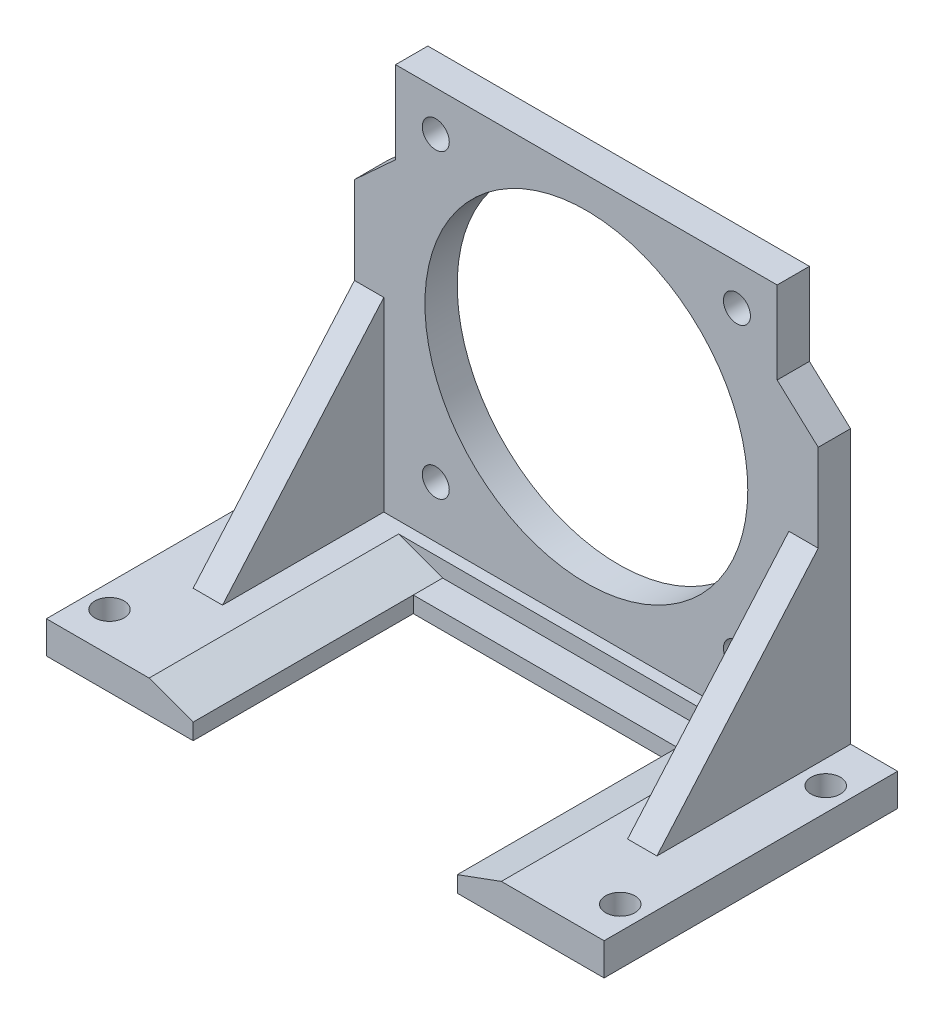
SolidWorks part; units mm, degrees
ref_plane "前视基准面" through (0, 0, 0) normal (0, 0, 1) x (1, 0, 0)
ref_plane "上视基准面" through (0, 0, 0) normal (0, 1, 0) x (1, 0, 0)
ref_plane "右视基准面" through (0, 0, 0) normal (1, 0, 0) x (0, 0, -1)
sketch "草图1" plane through (0, 0, 0) normal (0, 0, 1) x (1, 0, 0)
  line L0 (79, 24.1009) -> (79, 0)
  line L1 (65, -65) -> (-65, -65)
  line L2 (65, -65) -> (65, 65)
  line L3 (65, 65) -> (-65, 65)
  line L4 (-65, -65) -> (-65, 65)
  line L5 (65, -65) -> (-65, 65) construction
  line L6 (65, 65) -> (-65, -65) construction
  line L7 (-65, -65) -> (65, -65)
  line L8 (-65, -65) -> (-65, -69)
  line L9 (-65, -69) -> (65, -69)
  line L10 (65, -65) -> (65, -69)
  line L11 (-79, 0) -> (-79, -69)
  line L12 (-79, -69) -> (-65, -69)
  line L13 (0, 65) -> (0, -65) construction
  line L14 (79, -69) -> (65, -69)
  line L15 (65, 36.9502) -> (79, 24.1009)
  line L16 (79, 0) -> (79, -69)
  line L17 (-65, 36.9502) -> (-79, 24.1009)
  line L18 (-79, 24.1009) -> (-79, 0)
  circle A0 centre (0, -0.5) radius 55
  circle A1 centre (-51.3, 51.3) radius 4.6
  circle A2 centre (51.3, 51.3) radius 4.6
  circle A3 centre (51.3, -51.3) radius 4.6
  circle A4 centre (-51.3, -51.3) radius 4.6
  point P0 (0, 0)
  dimension "D3" = 68.5
  dimension "D4" = 9.2
  dimension "D5" = 102.6
  dimension "D6" = 4
  dimension "D8" = 110
  dimension "D1" = 130
  dimension "D2" = 130
  dimension "D7" = 158
extrude "凸台-拉伸1" add sketch "草图1" along normal mid plane 11
sketch "草图2" plane through (0, -69, 0) normal (0, -1, 0) x (1, 0, 0)
  line L0 (0, 31.1448) -> (0, -33.7851) construction
  line L1 (-95, -5.5432) -> (95, -5.5432)
  line L2 (-95, -5.5432) -> (-95, 94.4568)
  line L3 (-95, 94.4568) -> (-45, 94.4568)
  line L4 (95, -5.5432) -> (95, 94.4568)
  line L6 (-45, 94.4568) -> (-45, 19.4568)
  line L7 (-45, 19.4568) -> (45, 19.4568)
  line L8 (45, 94.4568) -> (45, 19.4568)
  line L9 (45, 94.4568) -> (95, 94.4568)
  circle A0 centre (-87, 80.9568) radius 5
  circle A1 centre (-87, 10.9568) radius 5
  circle A2 centre (87, 10.9568) radius 5
  circle A3 centre (87, 80.9568) radius 5
  dimension "D5" = 70
  dimension "D6" = 16.5
  dimension "D7" = 10
  dimension "D8" = 174
  dimension "D1" = 190
  dimension "D2" = 100
  dimension "D3" = 90
  dimension "D4" = 25
extrude "凸台-拉伸2" add sketch "草图2" along normal blind 11
ref_plane "基准面1" through (74, 0, 0) normal (1, 0, 0) x (0, 0, -1)
sketch "草图3" plane through (74, 0, 0) normal (1, 0, 0) x (0, 0, -1)
  line L0 (-5.5, -5.675) -> (-60.4568, -69)
  line L1 (-5.5, -69) -> (-5.5, -5.675)
  line L2 (5.5432, -69) -> (-94.4568, -69) construction
  line L3 (-60.4568, -69) -> (-5.5, -69)
  line L5 (-5.5, 24.1009) -> (-5.5, -69) construction
extrude "凸台-拉伸3" add sketch "草图3" along normal mid plane 10
mirror "镜向1" about plane through (0, 0, 0) normal (1, 0, 0) of "凸台-拉伸3"
sketch "草图4" plane through (0, 0, 94.4568) normal (0, 0, 1) x (1, 0, 0)
  line L0 (-60, -69) -> (-45, -74.5)
  line L1 (-45, -69) -> (-95, -69) construction
  line L2 (-45, -80) -> (-45, -69) construction
  line L3 (-45, -74.5) -> (45, -74.5)
  line L4 (45, -80) -> (45, -69) construction
  line L5 (0, -69) -> (0, -90.213) construction
  line L6 (69, -69) -> (-69, -69) construction
  line L7 (60, -69) -> (45, -74.5)
  line L8 (-60, -69) -> (60, -69)
  dimension "D1" = 120
extrude "切除-拉伸1" cut sketch "草图4" against normal blind 85
